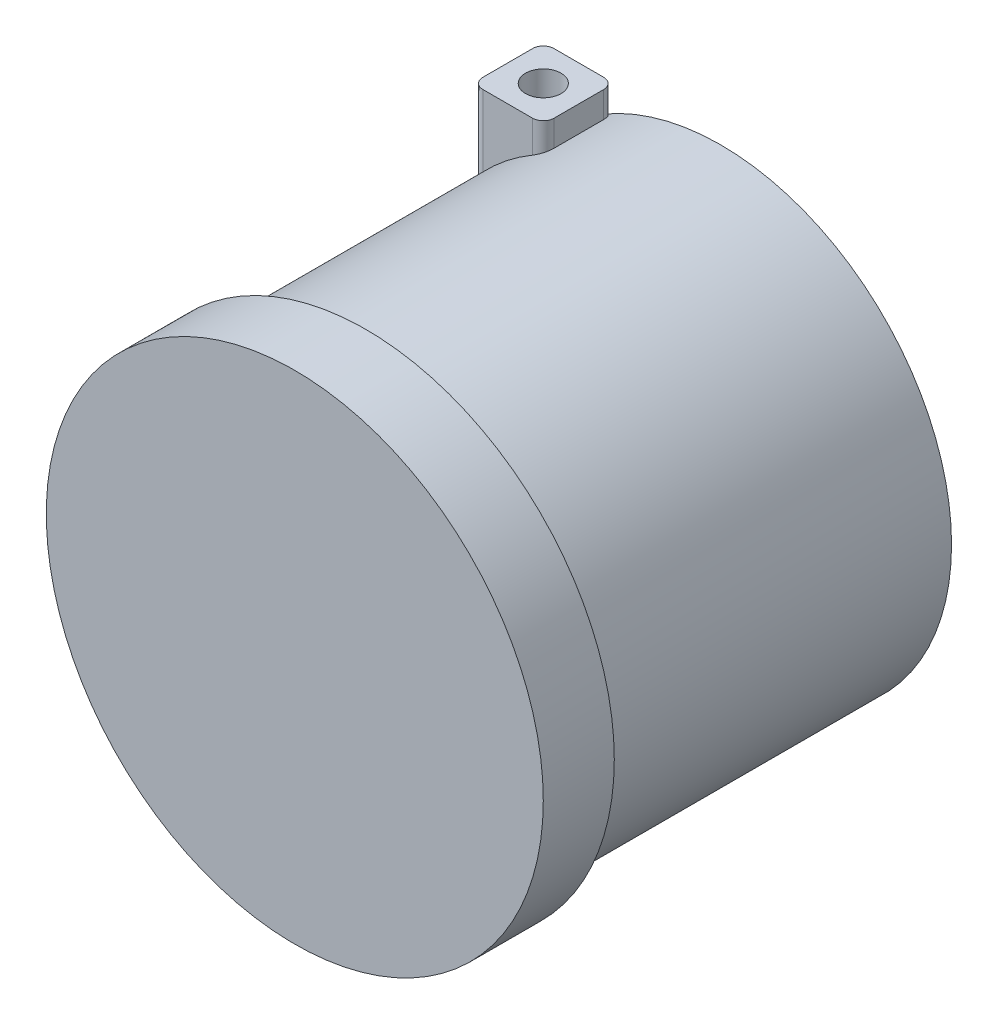
from build123d import *

# Parameters (mm, degrees)
SKETCH1_R           = 65
BOSS_EXTRUDE1_DEPTH = 100
SKETCH2_R           = 70
BOSS_EXTRUDE2_DEPTH = 20
SKETCH4_W           = 20
SKETCH4_H           = 24.089012679
BOSS_EXTRUDE4_DEPTH = 20
SKETCH5_R           = 5
CUT_EXTRUDE1_DEPTH  = 15
FILLET1_R           = 3


with BuildPart() as part:
    # Sketch1 → Boss-Extrude1 (new body)
    with BuildSketch(Plane.XY):
        Circle(SKETCH1_R)
    extrude(amount=BOSS_EXTRUDE1_DEPTH)

    # Sketch2 → Boss-Extrude2 (add)
    with BuildSketch(Plane.XY.offset(100)):
        Circle(SKETCH2_R)
    extrude(amount=BOSS_EXTRUDE2_DEPTH)

    # Sketch4 → Boss-Extrude4 (add)
    with BuildSketch(Plane(origin=(0, 0, 0), x_dir=(-1, 0, 0), z_dir=(0, 0, -1))):
        with Locations((40, 52.95549366)):
            Rectangle(SKETCH4_W, SKETCH4_H)
    extrude(amount=-BOSS_EXTRUDE4_DEPTH)

    # Sketch5 → Cut-Extrude1 (cut)
    with BuildSketch(Plane(origin=(0, 65, 0), x_dir=(1, 0, 0), z_dir=(0, 1, 0))):
        with Locations(Location((-40, -10, 0), (0, 0, 270))):
            Circle(SKETCH5_R)
    extrude(amount=-CUT_EXTRUDE1_DEPTH, mode=Mode.SUBTRACT)

    # Fillet1
    fillet1_edges = [part.edges().sort_by_distance(p)[0] for p in [
        (-30, 61.331406487, 20),
        (-50, 53.266559657, 20),
        (-30, 61.331406487, 0),
        (-50, 53.266559657, 0),
    ]]
    fillet(fillet1_edges, radius=FILLET1_R)


solid = part.part
